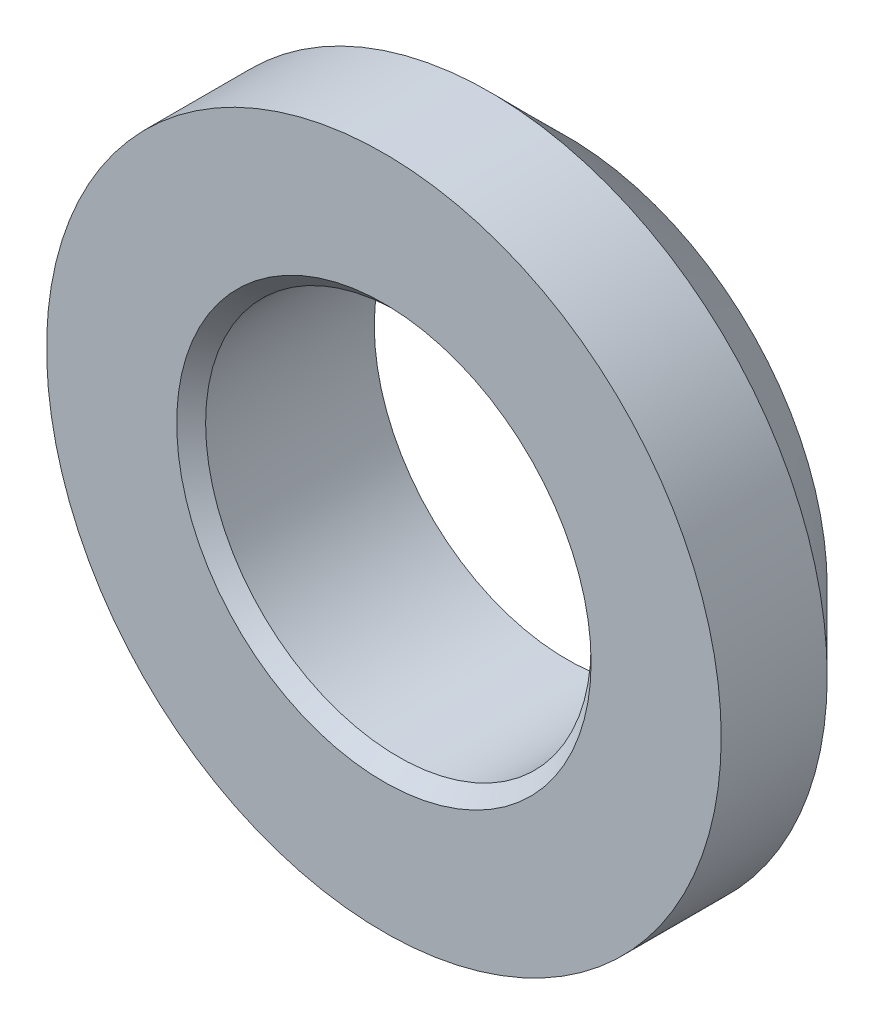
SolidWorks part; units mm, degrees
material "普通碳钢"
ref_plane "前视" through (0, 0, 0) normal (0, 0, 1) x (1, 0, 0)
ref_plane "上视" through (0, 0, 0) normal (0, 1, 0) x (1, 0, 0)
ref_plane "右视" through (0, 0, 0) normal (1, 0, 0) x (0, 0, -1)
sketch "草图1" plane through (0, 0, 0) normal (0, 0, 1) x (1, 0, 0)
  line L0 (-43.1325, 0) -> (47.5425, 0) construction
  line L1 (0, 28.3427) -> (0, -26.5141) construction
  circle A0 centre (0, 0) radius 20
  circle A1 centre (0, 0) radius 35
  dimension "D1" = 40
  dimension "D2" = 70
extrude "凸台-拉伸1" add sketch "草图1" along normal blind 19
chamfer "倒角1" distance 8 angle 45 1 edges at (35, 0, 0)
chamfer "倒角2" distance 1.5 angle 45 1 edges at (20, 0, 19)
